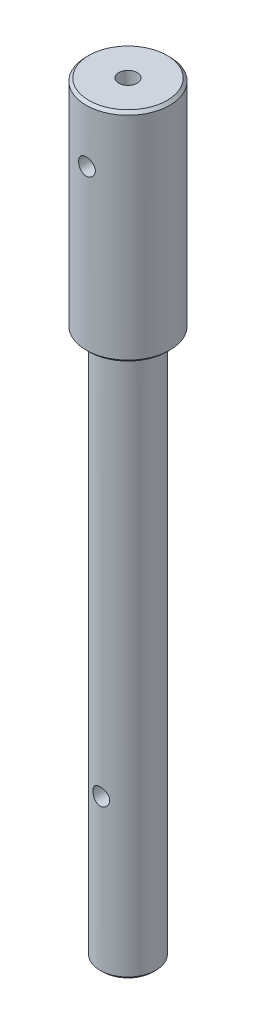
from build123d import *

# Parameters (mm, degrees)
M4_TAPPED_HOLE1_D     = 3.3
M4_TAPPED_HOLE1_DEPTH = 8.1
M4_TAPPED_HOLE1_TIP   = 0.991420021
SKETCH3_R             = 1.5
CUT_EXTRUDE1_DEPTH    = 8
M3_TAPPED_HOLE2_D     = 2.5
M3_TAPPED_HOLE2_DEPTH = 7.5
M3_TAPPED_HOLE2_TIP   = 0.751075774
CHAMFER1_SIZE         = 0.5
M3_TAPPED_HOLE3_D     = 2.5
M3_TAPPED_HOLE3_DEPTH = 7.5
M3_TAPPED_HOLE3_TIP   = 0.751075774
SKETCH9_R             = 1.5
CUT_EXTRUDE2_DEPTH    = 8


with BuildPart() as part:
    # Sketch1 → Revolve1 (revolve)
    with BuildSketch(Plane.XY, mode=Mode.PRIVATE) as revolve1_sk:
        Polygon((0, 0), (-7.5, 0), (-7.5, -39), (-5, -39), (-5, -136.5), (0, -136.5), align=None)
    revolve(revolve1_sk.sketch.rotate(Axis((0, 0, 0), (0, -1, 0)), 270), axis=Axis((0, 0, 0), (0, -1, 0)))

    # M4 Tapped Hole1
    with Locations(Plane.ZX):
        with Locations((0, 0)):
            Hole(M4_TAPPED_HOLE1_D / 2, depth=M4_TAPPED_HOLE1_DEPTH)
            with Locations((0, 0, -(M4_TAPPED_HOLE1_DEPTH + M4_TAPPED_HOLE1_TIP / 2))):  # 118° drill point
                Cone(0, M4_TAPPED_HOLE1_D / 2, M4_TAPPED_HOLE1_TIP, mode=Mode.SUBTRACT)

    # Sketch3 → Cut-Extrude1 (cut, symmetric)
    with BuildSketch(Plane.XY):
        with Locations((0, -10)):
            Circle(SKETCH3_R)
    extrude(amount=CUT_EXTRUDE1_DEPTH, both=True, mode=Mode.SUBTRACT)

    # M3 Tapped Hole2
    with Locations(Plane(origin=(0, -136.5, 0), x_dir=(0, 0, -1), z_dir=(0, -1, 0))):
        with Locations((0, 0)):
            Hole(M3_TAPPED_HOLE2_D / 2, depth=M3_TAPPED_HOLE2_DEPTH)
            with Locations((0, 0, -(M3_TAPPED_HOLE2_DEPTH + M3_TAPPED_HOLE2_TIP / 2))):  # 118° drill point
                Cone(0, M3_TAPPED_HOLE2_D / 2, M3_TAPPED_HOLE2_TIP, mode=Mode.SUBTRACT)

    # Chamfer1
    chamfer1_edges = [part.edges().sort_by_distance(p)[0] for p in [
        (0, -136.5, -5),
        (0, -39, -7.5),
        (0, 0, -7.5),
    ]]
    chamfer(chamfer1_edges, length=CHAMFER1_SIZE)

    # M3 Tapped Hole3
    with Locations(Plane(origin=(-7.5, -10, 0), x_dir=(0, 0, -1), z_dir=(-1, 0, 0))):
        with Locations((0, 0)):
            Hole(M3_TAPPED_HOLE3_D / 2, depth=M3_TAPPED_HOLE3_DEPTH)
            with Locations((0, 0, -(M3_TAPPED_HOLE3_DEPTH + M3_TAPPED_HOLE3_TIP / 2))):  # 118° drill point
                Cone(0, M3_TAPPED_HOLE3_D / 2, M3_TAPPED_HOLE3_TIP, mode=Mode.SUBTRACT)

    # Sketch9 → Cut-Extrude2 (cut, symmetric)
    with BuildSketch(Plane.XY):
        with Locations((0, -109)):
            Circle(SKETCH9_R)
    extrude(amount=CUT_EXTRUDE2_DEPTH, both=True, mode=Mode.SUBTRACT)


solid = part.part
